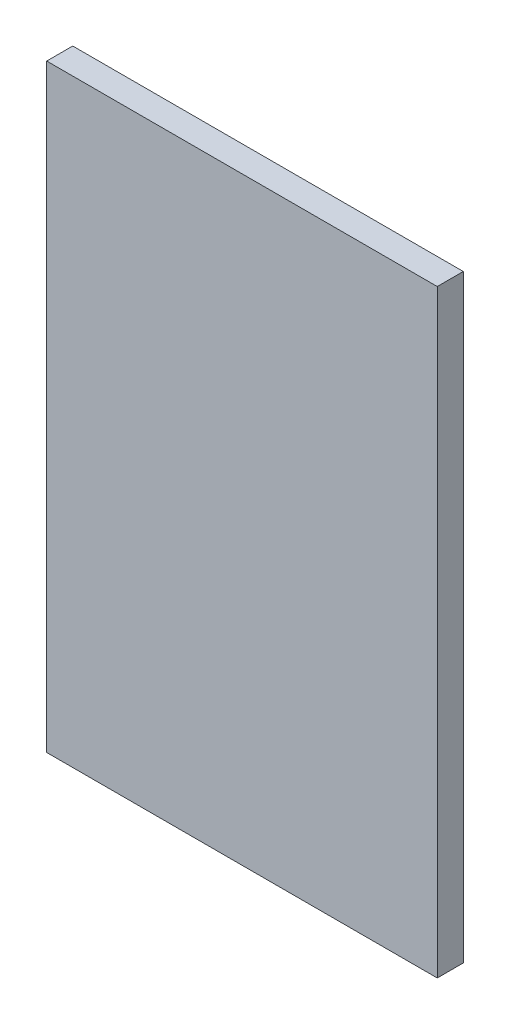
from build123d import *

# Parameters (mm, degrees)
SKETCH1_W           = 150
SKETCH1_H           = 230
BOSS_EXTRUDE1_DEPTH = 5


with BuildPart() as part:
    # Sketch1 → Boss-Extrude1 (new, symmetric)
    with BuildSketch(Plane.XY):
        Rectangle(SKETCH1_W, SKETCH1_H)
    extrude(amount=BOSS_EXTRUDE1_DEPTH, both=True)


solid = part.part
